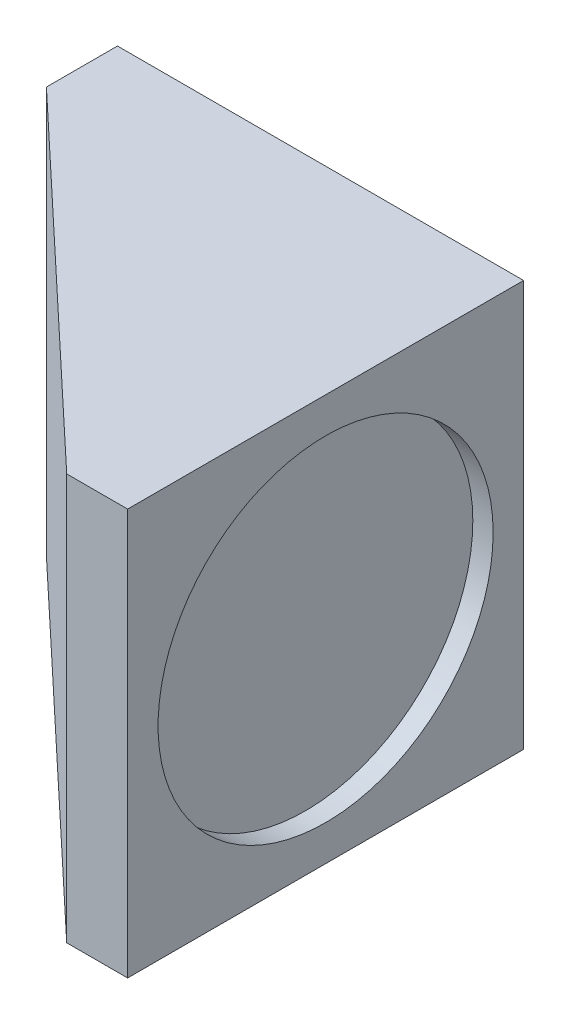
SolidWorks part; units mm, degrees
ref_plane "前视基准面" through (0, 0, 0) normal (0, 0, 1) x (1, 0, 0)
ref_plane "上视基准面" through (0, 0, 0) normal (0, 1, 0) x (1, 0, 0)
ref_plane "右视基准面" through (0, 0, 0) normal (1, 0, 0) x (0, 0, -1)
sketch "草图1" plane through (0, 0, 0) normal (0, 1, 0) x (1, 0, 0)
  line L0 (0, 0) -> (40, 0)
  line L1 (40, 0) -> (40, -39)
  line L2 (40, -39) -> (34, -39)
  line L3 (34, -39) -> (0, -7)
  line L4 (0, -7) -> (0, 0)
  dimension "D1" = 40
  dimension "D2" = 39
  dimension "D3" = 6
  dimension "D4" = 7
extrude "凸台-拉伸1" add sketch "草图1" along normal blind 40
sketch "草图2" plane through (40, 0, 0) normal (1, 0, 0) x (0, 0, -1)
  line L0 (0, 40) -> (0, 0) construction
  line L1 (-39, 0) -> (0, 0) construction
  circle A0 centre (-19.5, 20) radius 16.5
  dimension "D1" = 19.5
  dimension "D2" = 20
  dimension "D3" = 33
extrude "切除-拉伸1" cut sketch "草图2" against normal blind 2
